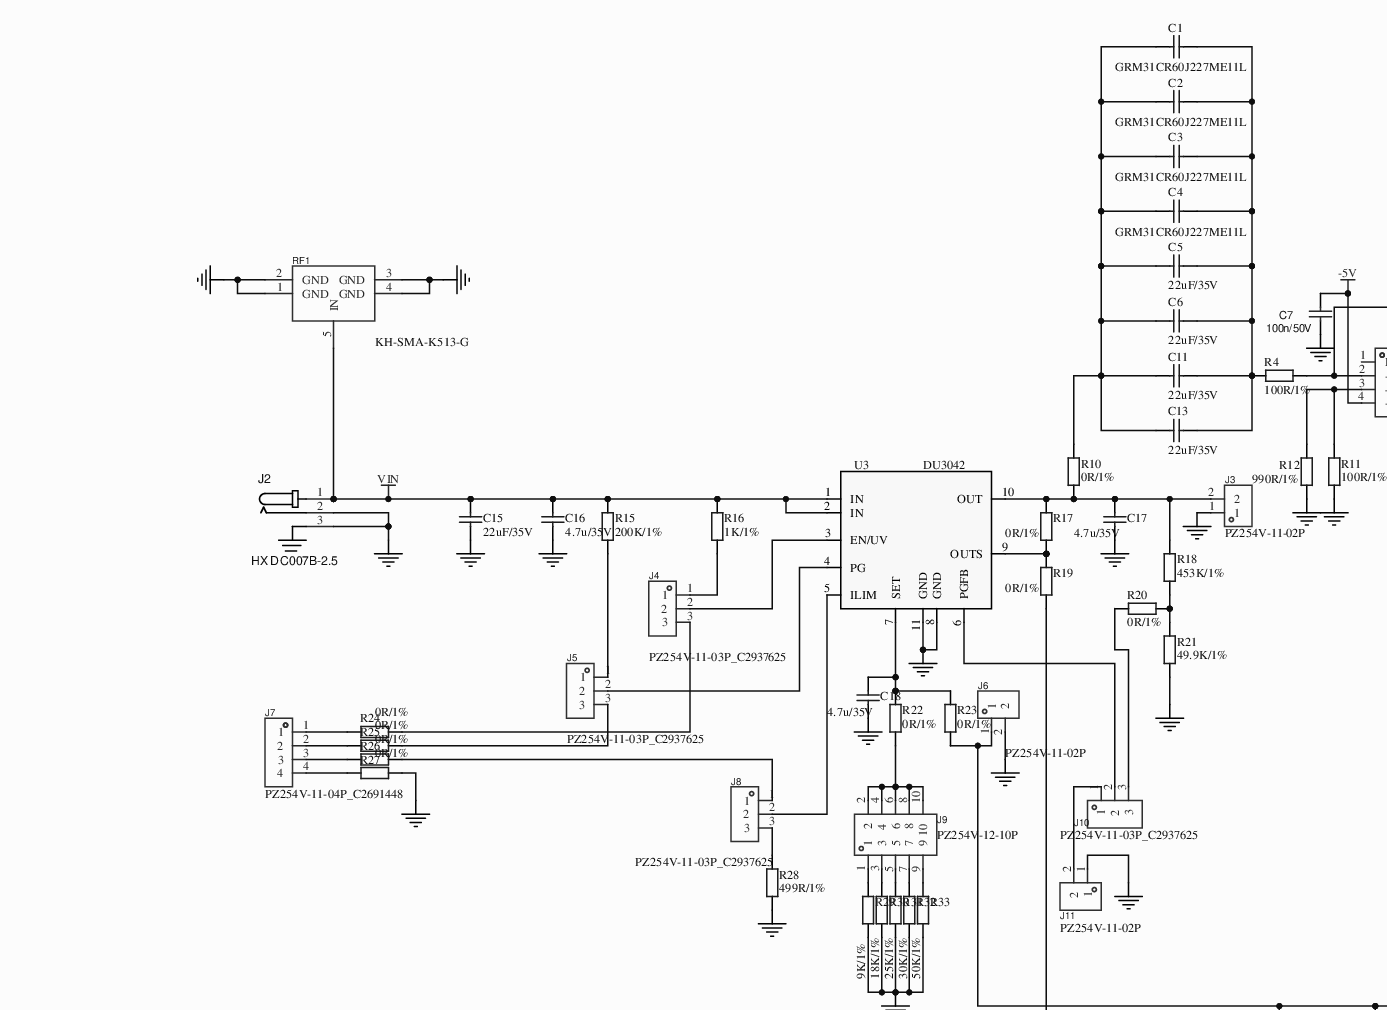
[diagram p0: MISC75514-2.SchDoc, top left]
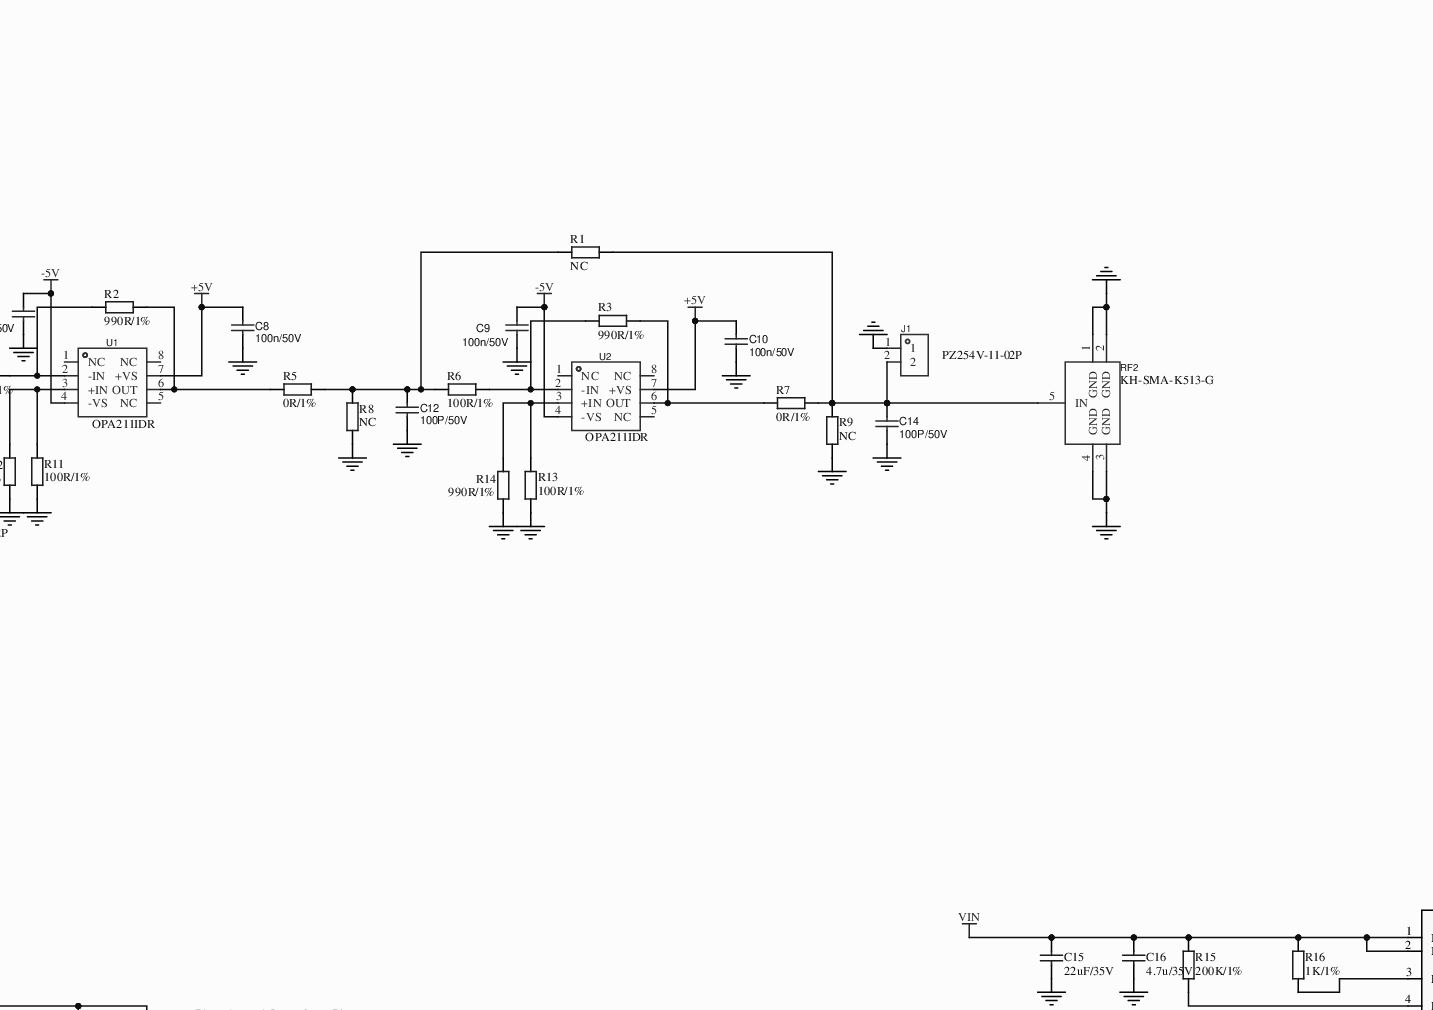
[diagram p1: MISC75514-2.SchDoc, top middle]
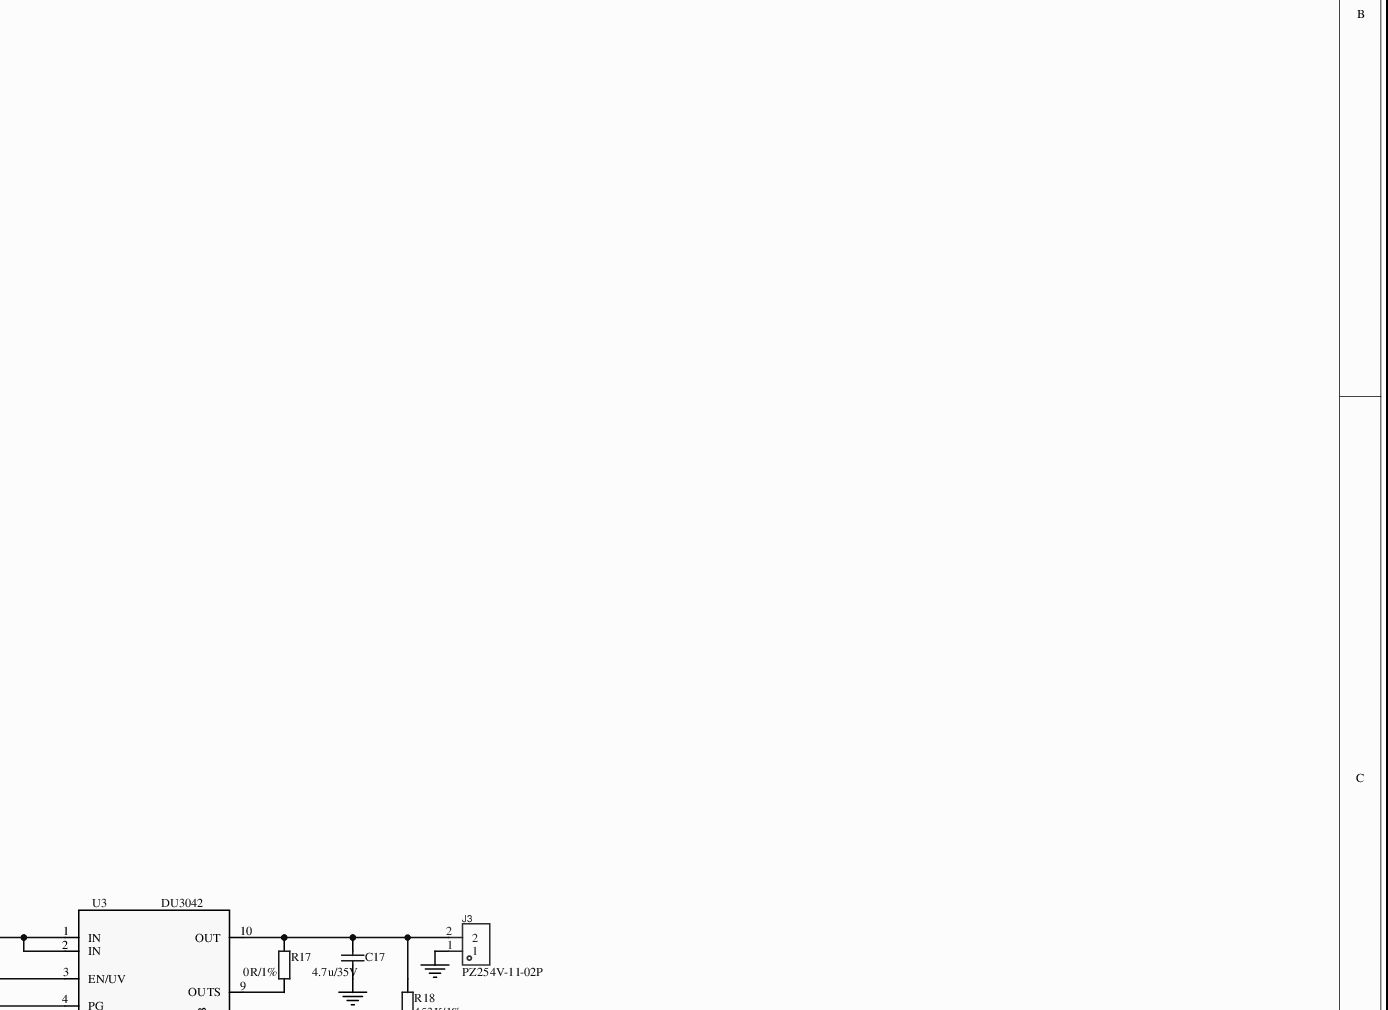
[diagram p2: MISC75514-2.SchDoc, top right]
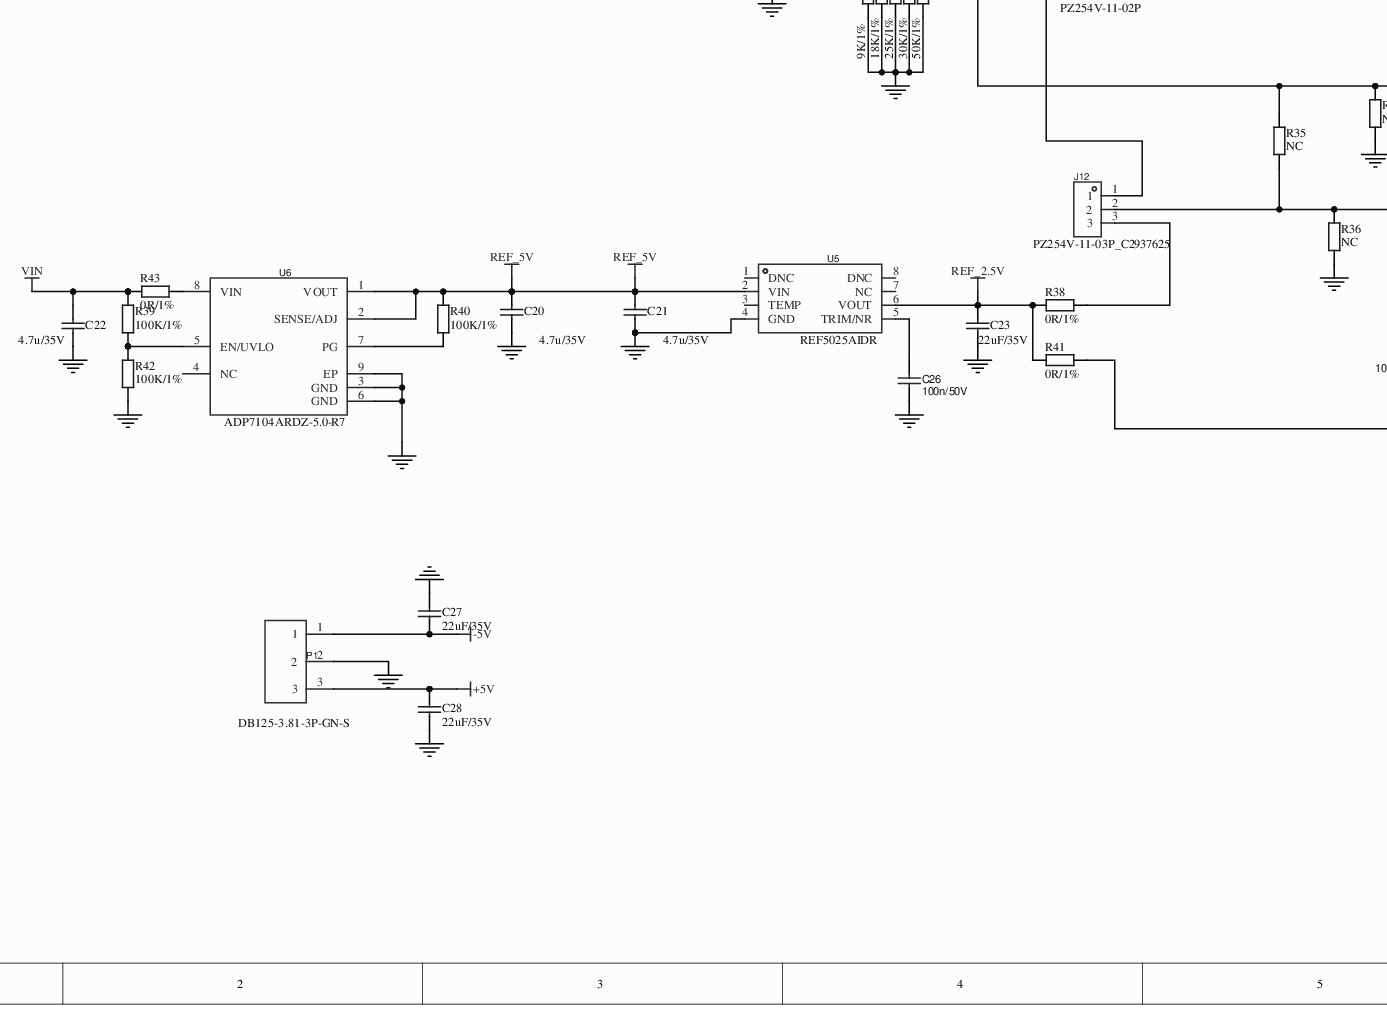
[diagram p3: MISC75514-2.SchDoc, bottom left]
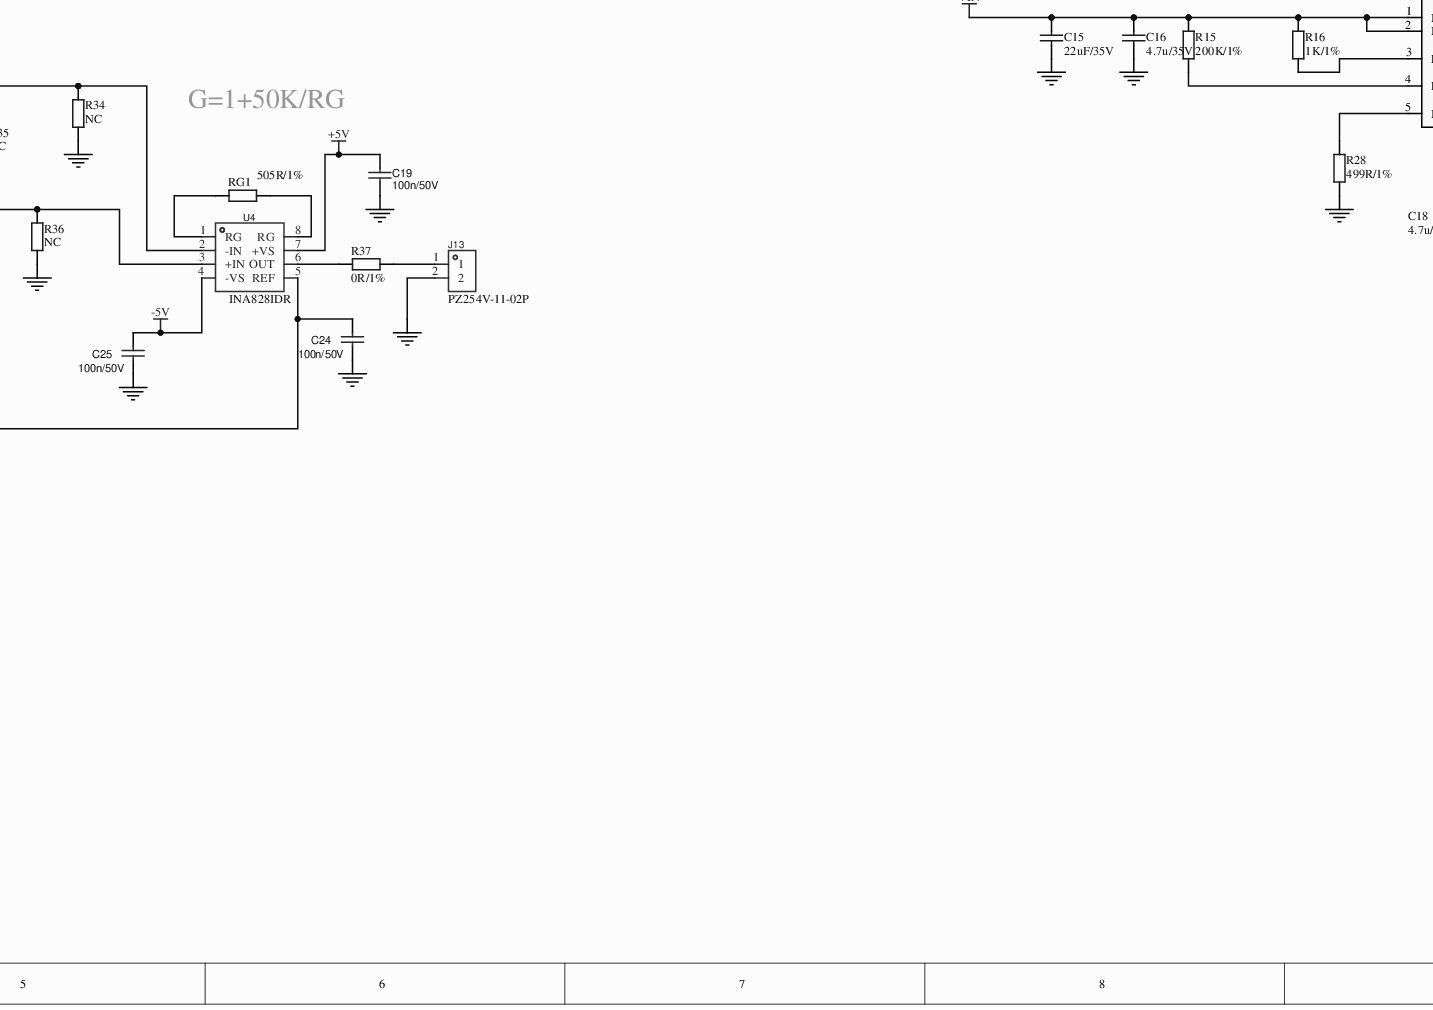
[diagram p4: MISC75514-2.SchDoc, bottom middle]
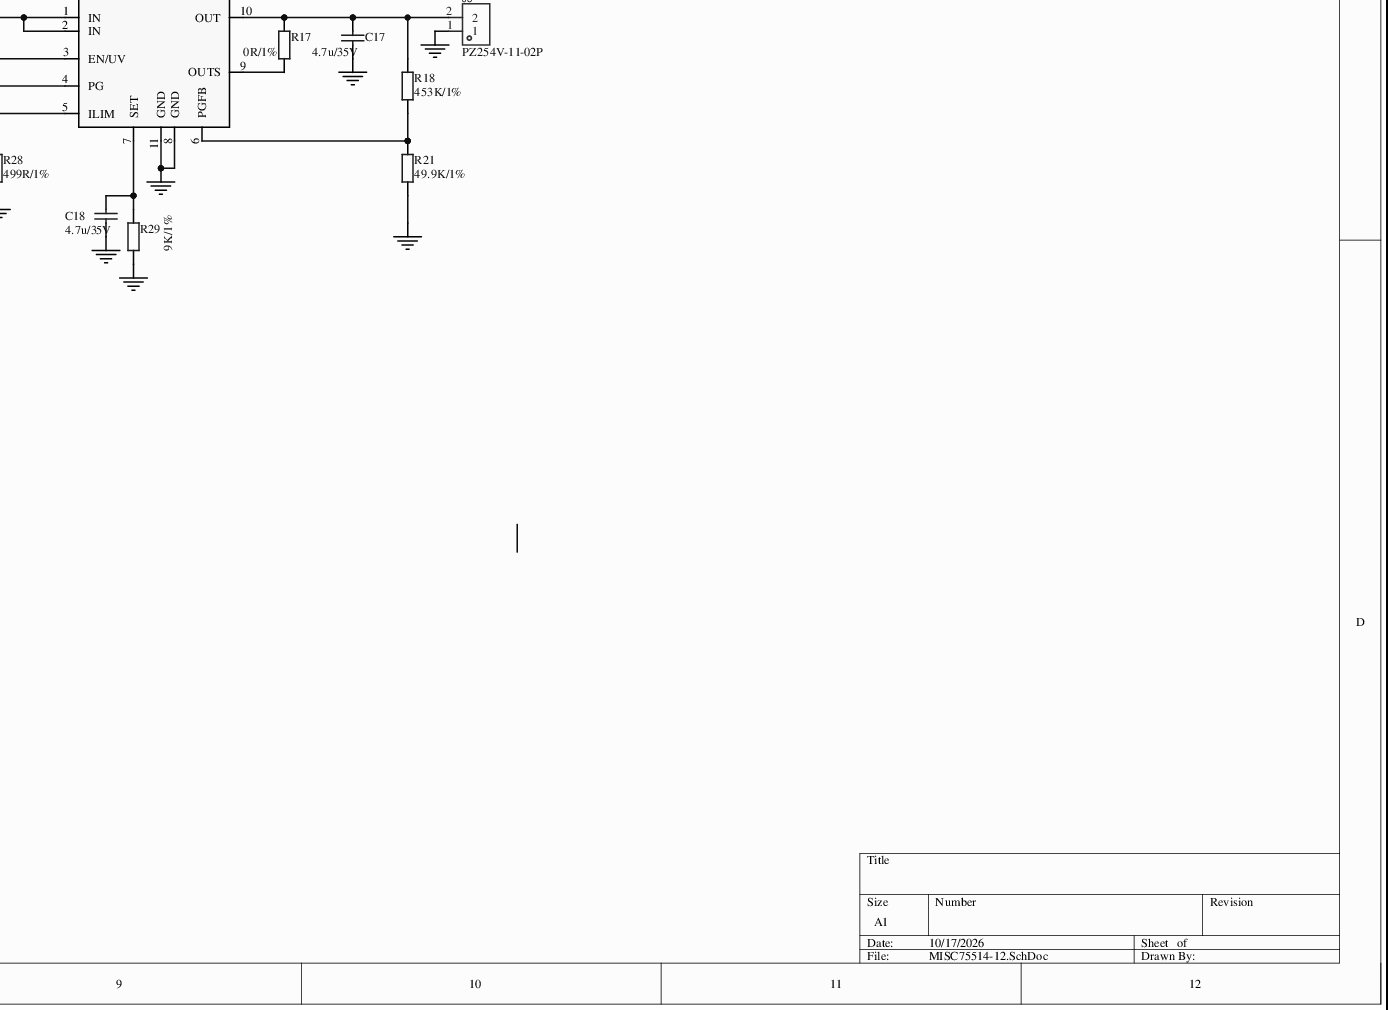
[diagram p5: MISC75514-2.SchDoc, bottom right]
# Altium schematic sheet MISC75514-2.SchDoc
size A2

## Parts
C1  GRM31CR60J227ME11L  [C1206]
C2  GRM31CR60J227ME11L  [C1206]
C3  GRM31CR60J227ME11L  [C1206]
C4  GRM31CR60J227ME11L  [C1206]
C5  22uF/35V  [C1206]
C6  22uF/35V  [C1206]
C7  100n/50V  [C0603]
C8  100n/50V  [C0603]
C9  100n/50V  [C0603]
C10  100n/50V  [C0603]
C11  22uF/35V  [C1206]
C12  100P/50V  [C0603]
C13  22uF/35V  [C1206]
C14  100P/50V  [C0603]
C15  22uF/35V  [C1206]
C16  4.7u/35V  [C0805]
C17  4.7u/35V  [C0805]
C18  4.7u/35V  [C0805]
C19  100n/50V  [C0603]
C20  4.7u/35V  [C0805]
C21  4.7u/35V  [C0805]
C22  4.7u/35V  [C0805]
C23  22uF/35V  [C1206]
C24  100n/50V  [C0603]
C25  100n/50V  [C0603]
C26  100n/50V  [C0603]
C27  22uF/35V  [C1206]
C28  22uF/35V  [C1206]
J1  PZ254V-11-02P  [HDR-TH_2P-P2.54-V-M]
J2  HX DC007B-2.5  [DC-IN-TH_HX-DC007B-2.5]
J3  PZ254V-11-02P  [HDR-TH_2P-P2.54-V-M]
J4  PZ254V-11-03P_C2937625  [HDR-TH_3P-P2.54-V-M]
J5  PZ254V-11-03P_C2937625  [HDR-TH_3P-P2.54-V-M]
J6  PZ254V-11-02P  [HDR-TH_2P-P2.54-V-M]
J7  PZ254V-11-04P_C2691448  [HDR-TH_4P-P2.54-V-M]
J8  PZ254V-11-03P_C2937625  [HDR-TH_3P-P2.54-V-M]
J9  PZ254V-12-10P  [HDR-TH_10P-P2.54-V-M-R2-C5-S2.54]
J10  PZ254V-11-03P_C2937625  [HDR-TH_3P-P2.54-V-M]
J11  PZ254V-11-02P  [HDR-TH_2P-P2.54-V-M]
J12  PZ254V-11-03P_C2937625  [HDR-TH_3P-P2.54-V-M]
J13  PZ254V-11-02P  [HDR-TH_2P-P2.54-V-M]
P1  DB125-3.81-3P-GN-S  [CONN-TH_3P-P3.81_L7.4-W11.4]
R1  NC  [R0603]
R2  990R/1%  [R0603]
R3  990R/1%  [R0603]
R4  100R/1%  [R0603]
R5  0R/1%  [R0603]
R6  100R/1%  [R0603]
R7  0R/1%  [R0603]
R8  NC  [R0603]
R9  NC  [R0603]
R10  0R/1%  [R0603]
R11  100R/1%  [R0603]
R12  990R/1%  [R0603]
R13  100R/1%  [R0603]
R14  990R/1%  [R0603]
R15  200K/1%  [R0603]
R16  1K/1%  [R0603]
R17  0R/1%  [R0603]
R18  453K/1%  [R0603]
R19  0R/1%  [R0603]
R20  0R/1%  [R0603]
R21  49.9K/1%  [R0603]
R22  0R/1%  [R0603]
R23  0R/1%  [R0603]
R24  0R/1%  [R0603]
R25  0R/1%  [R0603]
R26  0R/1%  [R0603]
R27  0R/1%  [R0603]
R28  499R/1%  [R0603]
R29  9K/1%  [R0603]
R30  18K/1%  [R0603]
R31  25K/1%  [R0603]
R32  30K/1%  [R0603]
R33  50K/1%  [R0603]
R34  NC  [R0603]
R35  NC  [R0603]
R36  NC  [R0603]
R37  0R/1%  [R0603]
R38  0R/1%  [R0603]
R39  100K/1%  [R0603]
R40  100K/1%  [R0603]
R41  0R/1%  [R0603]
R42  100K/1%  [R0603]
R43  0R/1%  [R0603]
RF1  KH-SMA-K513-G  [ANT-TH_KH-SMA-K513-G]
RF2  KH-SMA-K513-G  [ANT-TH_KH-SMA-K513-G]
RG1  505R/1%  [R0603]
U1  OPA211IDR  [SOIC-8_L5.0-W4.0-P1.27-LS6.0-BL]
U2  OPA211IDR  [SOIC-8_L5.0-W4.0-P1.27-LS6.0-BL]
U3  DU3042  [WSON-10_L3.0-W3.0-P0.50-BL-EP]
U4  INA828IDR  [SOIC-8_L5.0-W4.0-P1.27-LS6.0-BL]
U5  REF5025AIDR  [SOIC-8_L5.0-W4.0-P1.27-LS6.0-BL]
U6  ADP7104ARDZ-5.0-R7  [SOIC-8_L4.9-W3.9-P1.27-LS6.0-BL-EP]

## Nets
+5V: C8.1 C10.1 C19.1 C28.2 P1.3 U1.7(+VS) U2.7(+VS) U4.7(+VS)
-5V: C7.1 C9.1 C25.1 C27.2 P1.1 U1.4(-VS) U2.4(-VS) U4.4(-VS)
GND: C7.2 C8.2 C9.2 C10.2 C12.2 C14.2 C15.1 C16.1 C17.1 C18.1 C19.2 C20.1 C21.1 C22.1 C23.2 C24.2 C25.2 C26.2 C27.1 C28.1 J1.1 J2.2 J2.3 J3.1 J6.2 J11.1 J13.2 P1.2 R8.1 R9.1 R11.1 R12.1 R13.1 R14.1 R21.2 R27.1 R28.1 R29.1 R30.1 R31.1 R32.1 R33.1 R34.2 R36.2 R42.1 RF1.1(GND) RF1.2(GND) RF1.3(GND) RF1.4(GND) RF2.1(GND) RF2.2(GND) RF2.3(GND) RF2.4(GND) U3.8(GND) U3.11(GND) U5.4(GND) U6.3(GND) U6.6(GND) U6.9(EP)
REF_2.5V: C23.1 R38.1 R41.1 U5.6(VOUT)
REF_5V: C20.2 C21.2 R40.2 U5.2(VIN) U6.1(VOUT) U6.2(SENSE/ADJ)
VIN: C15.2 C16.2 C22.2 J2.1 R15.2 R16.2 R39.2 R43.1 RF1.5(IN) U3.1(IN) U3.2(IN)
NetC1_1: C1.1 C2.1 C3.1 C4.1 C5.1 C6.1 C11.1 C13.1 R4.1
NetC1_2: C1.2 C2.2 C3.2 C4.2 C5.2 C6.2 C11.2 C13.2 R10.1
NetC12_1: C12.1 R1.2 R5.2 R6.1 R8.2
NetC14_1: C14.1 J1.2 R1.1 R7.2 R9.2 RF2.5(IN)
NetC17_2: C17.2 J3.2 R10.2 R17.1 R18.1 U3.10(OUT)
NetC18_2: C18.2 R22.1 R23.1 U3.7(SET)
NetC24_1: C24.1 R41.2 U4.5(REF)
NetC26_1: C26.1 U5.5(TRIM/NR)
NetJ4_1: J4.1 R16.1
NetJ4_2: J4.2 U3.3(EN/UV)
NetJ4_3: J4.3 R24.1
NetJ5_1: J5.1 R15.1
NetJ5_2: J5.2 U3.4(PG)
NetJ5_3: J5.3 R25.1
NetJ6_1: J6.1 R23.2 R34.1 R35.1 U4.2(-IN)
NetJ7_1: J7.1 R24.2
NetJ7_2: J7.2 R25.2
NetJ7_3: J7.3 R26.2
NetJ7_4: J7.4 R27.2
NetJ8_1: J8.1 R26.1
NetJ8_2: J8.2 U3.5(ILIM)
NetJ8_3: J8.3 R28.2
NetJ9_1: J9.1 R29.2
NetJ9_2: J9.2 J9.4 J9.6 J9.8 J9.10 R22.2
NetJ9_3: J9.3 R30.2
NetJ9_5: J9.5 R31.2
NetJ9_7: J9.7 R32.2
NetJ9_9: J9.9 R33.2
NetJ10_1: J10.1 J11.2
NetJ10_2: J10.2 U3.6(PGFB)
NetJ10_3: J10.3 R20.1
NetJ12_1: J12.1 R19.2
NetJ12_2: J12.2 R35.2 R36.1 U4.3(+IN)
NetJ12_3: J12.3 R38.2
NetJ13_1: J13.1 R37.2
NetR2_1: R2.1 R5.1 U1.6(OUT)
NetR2_2: R2.2 R4.2 U1.2(-IN)
NetR3_1: R3.1 R7.1 U2.6(OUT)
NetR3_2: R3.2 R6.2 U2.2(-IN)
NetR11_2: R11.2 R12.2 U1.3(+IN)
NetR13_2: R13.2 R14.2 U2.3(+IN)
NetR17_2: R17.2 R19.1 U3.9(OUTS)
NetR18_2: R18.2 R20.2 R21.1
NetR37_1: R37.1 U4.6(OUT)
NetR39_1: R39.1 R42.2 U6.5(EN/UVLO)
NetR40_1: R40.1 U6.7(PG)
NetR43_2: R43.2 U6.8(VIN)
NetRG1_1: RG1.1 U4.8(RG)
NetRG1_2: RG1.2 U4.1(RG)

Not connected (* = marked no-connect by the designer): U1 1(NC) 5(NC) 8(NC); U2 1(NC) 5(NC) 8(NC); U5 1(DNC) 3(TEMP) 7(NC) 8(DNC); U6 4(NC)

## Notes on the sheet
- G=1+50K/RG

## Library data of the parts
C1-C6 C11 C13 C15-C18 C20-C23 C27 C28 = C: SMD capacitor; BOM名称: Non-polar SMD capacitor
C7-C10 C12 C14 C19 C24-C26 = 1uF: Manufacturer Part: CL10A105KB8NNNC; nameAlias: Value; Supplier: LCSC; Supplier Part: C15849; JLCPCB Part Class: Basic Part; spicePre: C; spiceSymbolName: CL10A105KB8NNNC
J2 = HX DC007B-2.5: Manufacturer: hanxia(韩下); Add into BOM: yes; Connector Type: DC power jack; Inside Contact Diameter: 2.5mm; Outside Contact Diameter: 6.4mm; Current Rating (Max): 7A; Voltage Rating (Max): 20V; Name: HX DC007B-2.5; Symbol: HX DC007B-2.5; Device: HX DC007B-2.5; Supplier: LCSC; Supplier Part: C19189083; Manufacturer Part: HX DC007B-2.5; LCSC Part Name: DC电源插座 内径:2.5mm 外径:6.4mm; Supplier Footprint: 插件; Datasheet: https://atta.szlcsc.com/upload/public/pdf/source/20231103/814B3421283469BAAEFFF9B7A53EC0CB.pdf; Convert to PCB: yes; Mounting Style: Right angle THT; Operating Temperature Range: -25℃~+70℃
P1 = WJ124-3.81-3P: Symbol: WJ124-3.81-3P
R1-R43 RG1 = R: SMD resistor; BOM名称: SMD resistor
U1 U2 = INA828IDR: Symbol: INA828IDR
U3 = DAC53202RTER: No Description Available; Mfr_Name: Texas Instruments; Type: Data Acquisition; RefDes: RefDes
J1 J3 J6 J11 J13 = PZ254V-11-02P: Symbol: PZ254V-11-02P
J4 J5 J8 J10 J12 = PZ254V-11-03P_C2937625: Symbol: PZ254V-11-03P_C2937625
J7 = PZ254V-11-04P_C2691448: Symbol: PZ254V-11-04P_C2691448
J9 = PZ254V-12-10P: Symbol: PZ254V-12-10P
RF1 RF2 = KH-SMA-K513-G: Symbol: KH-SMA-K513-G
U4 = INA828IDR: Symbol: INA828IDR
U5 = REF5025AIDR: Symbol: REF5025AIDR
U6 = ADP7104ARDZ-5.0-R7: Symbol: ADP7104ARDZ-5.0-R7